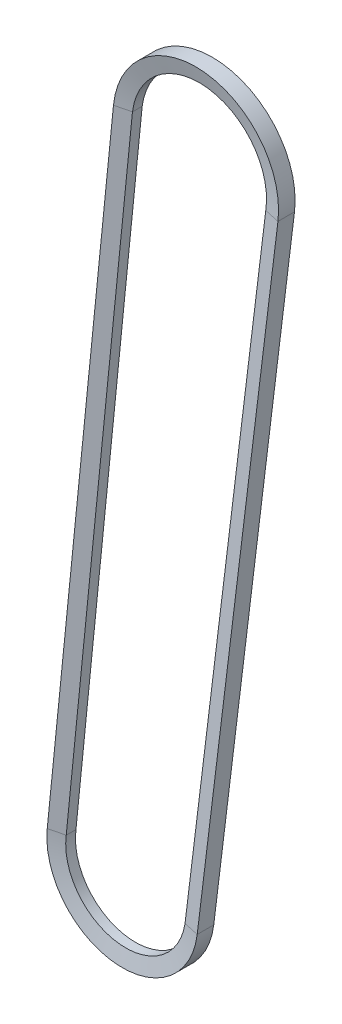
from build123d import *


with BuildPart() as part:
    # 扫描1: sweep along a path in 草图1
    with BuildLine(Plane.XY) as sweep_1_path:
        Line((133.935000245, 322.9682066), (50.990864547, -352.799410804))
        ThreePointArc((50.990864547, -352.799410804), (-34.525526627, -420.379935429), (-103.043927412, -335.613142274))
        Line((-103.043927412, -335.613142274), (-35.006384485, 341.817662407))
        ThreePointArc((-35.006384485, 341.817662407), (58.993428728, 417.799266002), (133.935000245, 322.9682066))
    # 草图2 → 扫描1 (sweep)
    with BuildSketch(Plane(origin=(0, 322.9682066, 0), x_dir=(1, 0, 0), z_dir=(0, 1, 0))):
        Polygon((133.935000245, 8.5), (133.935000245, -8.5), (117.935000245, -5), (117.935000245, 5), align=None)
    sweep(path=sweep_1_path.line)


solid = part.part
